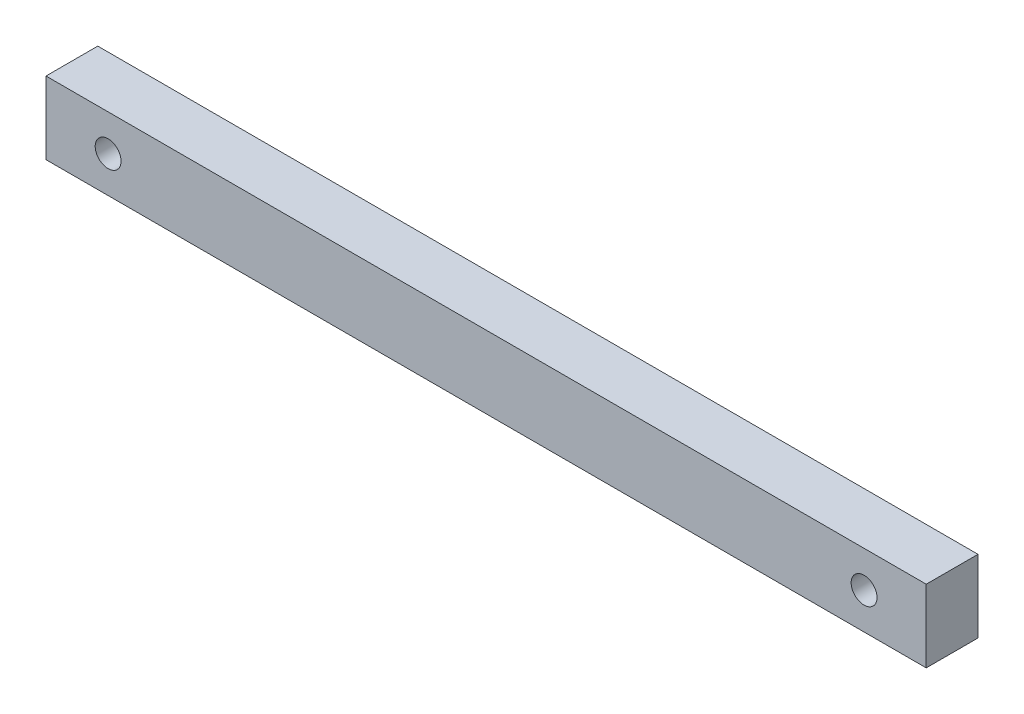
from build123d import *

# Parameters (mm, degrees)
SKETCH_1_W                   = 170
SKETCH_1_H                   = 14
EXTRUDE_1_DEPTH              = 5
HOLE_WIZARD_M6_1_D           = 5
HOLE_WIZARD_M6_1_CSINK_D     = 6.05
HOLE_WIZARD_M6_1_CSINK_ANGLE = 90


with BuildPart() as part:
    # 草图1 → 凸台-拉伸1 (new, symmetric)
    with BuildSketch(Plane.XY):
        Rectangle(SKETCH_1_W, SKETCH_1_H)
    extrude(amount=EXTRUDE_1_DEPTH, both=True)

    # M6 螺纹孔1 (through all)
    with Locations(Plane(origin=(-73, 0, -5), x_dir=(-1, 0, 0), z_dir=(0, 0, -1))):
        with Locations((0, 0)):
            hole_wizard_m6_1 = CounterSinkHole(HOLE_WIZARD_M6_1_D / 2, HOLE_WIZARD_M6_1_CSINK_D / 2, counter_sink_angle=HOLE_WIZARD_M6_1_CSINK_ANGLE)

    # 镜向1: M6 螺纹孔1 across plane
    add(hole_wizard_m6_1.mirror(Plane(origin=(0, 0, 0), x_dir=(0, 0, 1), z_dir=(1, 0, 0))), mode=Mode.SUBTRACT)


solid = part.part
